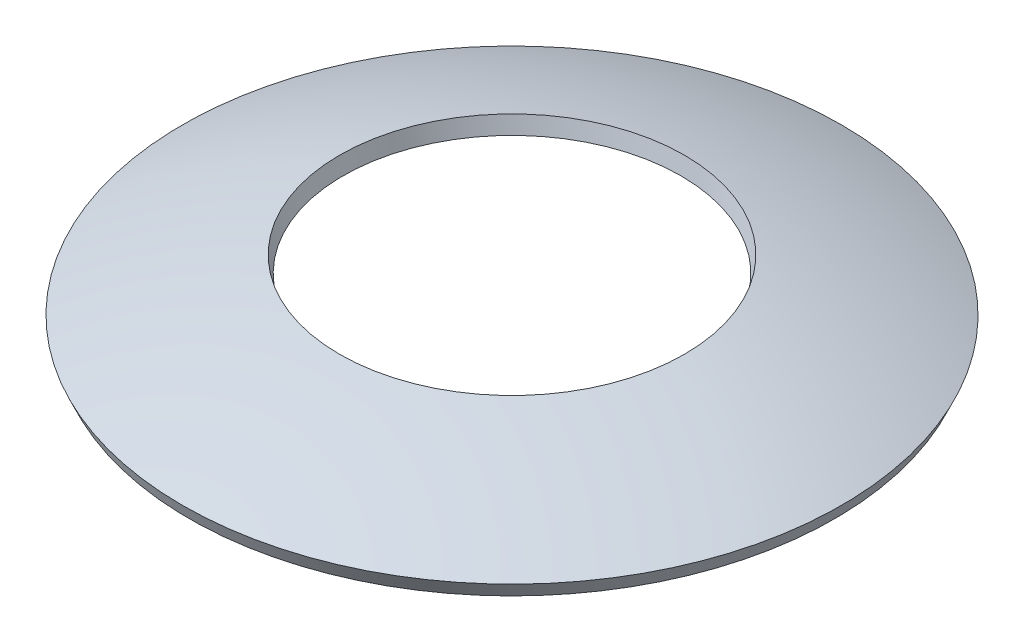
from build123d import *


with BuildPart() as part:
    # Sketch1 → Revolve1 (revolve)
    with BuildSketch(Plane(origin=(0, 0, 0), x_dir=(0, 0, -1), z_dir=(1, 0, 0))):
        with BuildLine():
            Line((32.25, 46.380895852), (32.465789474, 47.357335764))
            ThreePointArc((32.465789474, 47.357335764), (37.31529182, 46.018385852), (42, 44.18427322))
            Line((42, 44.18427322), (41.587628866, 43.273257278))
            ThreePointArc((41.587628866, 43.273257278), (36.999512608, 45.069553154), (32.25, 46.380895852))
        make_face()
    revolve(axis=Axis((0, 0, -22), (0, 1, 0)))


solid = part.part
